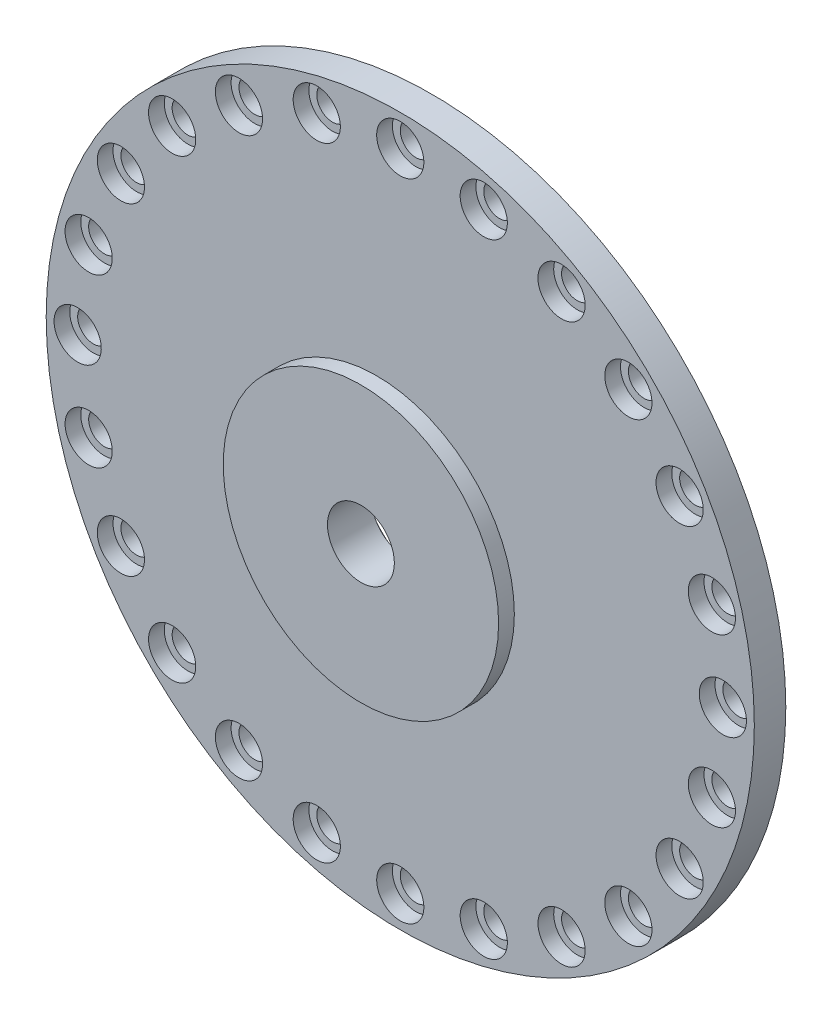
from build123d import *

# Parameters (mm, degrees)
SKETCH_1_R               = 450
SKETCH_1_R_2             = 42.5
EXTRUDE_1_DEPTH          = 20
PATTERN_CIRCULAR_1_COUNT = 24
SKETCH_7_R               = 125
SKETCH_7_R_2             = 42.5
EXTRUDE_2_DEPTH          = 30
SKETCH_8_R               = 175
SKETCH_8_R_2             = 42.5
EXTRUDE_3_DEPTH          = 20
SKETCH_9_R               = 90
CUT_EXTRUDE_1_DEPTH      = 34


with BuildPart() as part:
    # 草图1 → 凸台-拉伸1 (new, symmetric)
    with BuildSketch(Plane.XY):
        Circle(SKETCH_1_R)
        Circle(SKETCH_1_R_2, mode=Mode.SUBTRACT)
    extrude(amount=EXTRUDE_1_DEPTH, both=True)

    # 草图4 → M42 六角头螺栓的柱形沉头孔1 (revolve, cut)
    with BuildSketch(Plane(origin=(0, 410, 20), x_dir=(0, -1, 0), z_dir=(1, 0, 0))):
        Polygon((0, 0), (0, 62.017212381), (20, 50), (20, 20), (30, 20), (30, 0), align=None)
    hole_wizard_m42_1 = revolve(axis=Axis((0, 410, 26.35), (0, 0, -1)), mode=Mode.SUBTRACT)

    # 阵列(圆周)1: M42 六角头螺栓的柱形沉头孔1 ×24 about axis
    pattern_circular_1_axis = Axis((0, 0, 0), (0, 0, 1))
    for i in range(1, PATTERN_CIRCULAR_1_COUNT):
        add(hole_wizard_m42_1.rotate(pattern_circular_1_axis, i * 360 / PATTERN_CIRCULAR_1_COUNT), mode=Mode.SUBTRACT)

    # 草图7 → 凸台-拉伸2 (add)
    with BuildSketch(Plane.XY.offset(20)):
        Circle(SKETCH_7_R)
        Circle(SKETCH_7_R_2, mode=Mode.SUBTRACT)
    extrude(amount=EXTRUDE_2_DEPTH)

    # 草图8 → 凸台-拉伸3 (add)
    with BuildSketch(Plane.XY.offset(50)):
        Circle(SKETCH_8_R)
        Circle(SKETCH_8_R_2, mode=Mode.SUBTRACT)
    extrude(amount=EXTRUDE_3_DEPTH)

    # 草图9 → 切除-拉伸1 (cut)
    with BuildSketch(Plane(origin=(0, 0, -20), x_dir=(-1, 0, 0), z_dir=(0, 0, -1))):
        Circle(SKETCH_9_R)
    extrude(amount=-CUT_EXTRUDE_1_DEPTH, mode=Mode.SUBTRACT)


solid = part.part
